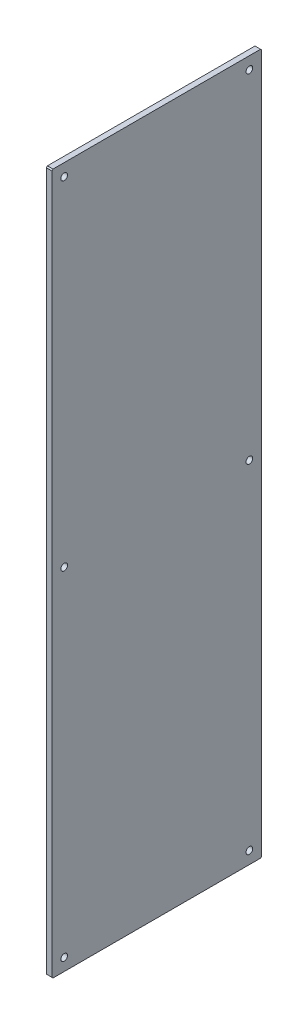
SolidWorks part; units mm, degrees
material "PC(透明)"
ref_plane "前基準面" through (0, 0, 0) normal (0, 0, 1) x (1, 0, 0)
ref_plane "上基準面" through (0, 0, 0) normal (0, 1, 0) x (1, 0, 0)
ref_plane "右基準面" through (0, 0, 0) normal (1, 0, 0) x (0, 0, -1)
sketch "草图1" plane through (0, 0, 0) normal (1, 0, 0) x (0, 0, -1)
  line L1 (94, 314) -> (-94, 314)
  line L2 (94, 314) -> (94, -314)
  line L3 (94, -314) -> (-94, -314)
  line L4 (-94, 314) -> (-94, -314)
  line L5 (94, 314) -> (-94, -314) construction
  line L6 (94, -314) -> (-94, 314) construction
  point P0 (0, 0)
  dimension "D1" = 188
  dimension "D2" = 628
extrude "凸台-拉伸1" add sketch "草图1" along normal blind 5
chamfer "倒角1" distance 1 angle 45 4 edges at (2.5, -314, -94) (2.5, -314, 94) (2.5, 314, -94) (2.5, 314, 94)
sketch "草图2" plane through (0, 0, 0) normal (-1, 0, 0) x (0, 0, 1)
  line L0 (-94, -313) -> (-94, 313) construction
  line L1 (-93, 314) -> (93, 314) construction
  line L2 (58.8862, 0) -> (0, 0) construction
  line L3 (0, 0) -> (0, 69.8386) construction
  line L5 (83, -303) -> (-83, -303) construction
  line L6 (83, -303) -> (83, 303) construction
  line L7 (83, 303) -> (-83, 303) construction
  line L8 (-83, -303) -> (-83, 303) construction
  line L9 (83, -303) -> (-83, 303) construction
  line L10 (83, 303) -> (-83, -303) construction
  circle A0 centre (-83, 303) radius 3
  circle A1 centre (-83, -303) radius 3
  circle A2 centre (83, -303) radius 3
  circle A3 centre (83, 303) radius 3
  circle A8 centre (83, 0) radius 3
  circle A9 centre (-83, 0) radius 3
  dimension "D1" = 6
  dimension "D2" = 11
  dimension "D3" = 11
extrude "切除-拉伸1" cut sketch "草图2" against normal through all
sketch "草图3" plane through (5, 0, 0) normal (1, 0, 0) x (0, 0, -1)
  line L0 (-74, -254) -> (-94, -254) construction
  line L2 (-74, -264) -> (-94, -264)
  line L3 (-74, -244) -> (-94, -244)
  line L4 (-93, -314) -> (93, -314) construction
  line L5 (-94, 313) -> (-94, -313) construction
  arc A0 (-74, -264) -> (-74, -244) centre (-74, -254) ccw
  arc A1 (-94, -244) -> (-94, -264) centre (-94, -254) ccw
  point P4 (-84, -254)
  dimension "D1" = 20
  dimension "D2" = 60
  dimension "D3" = 20
